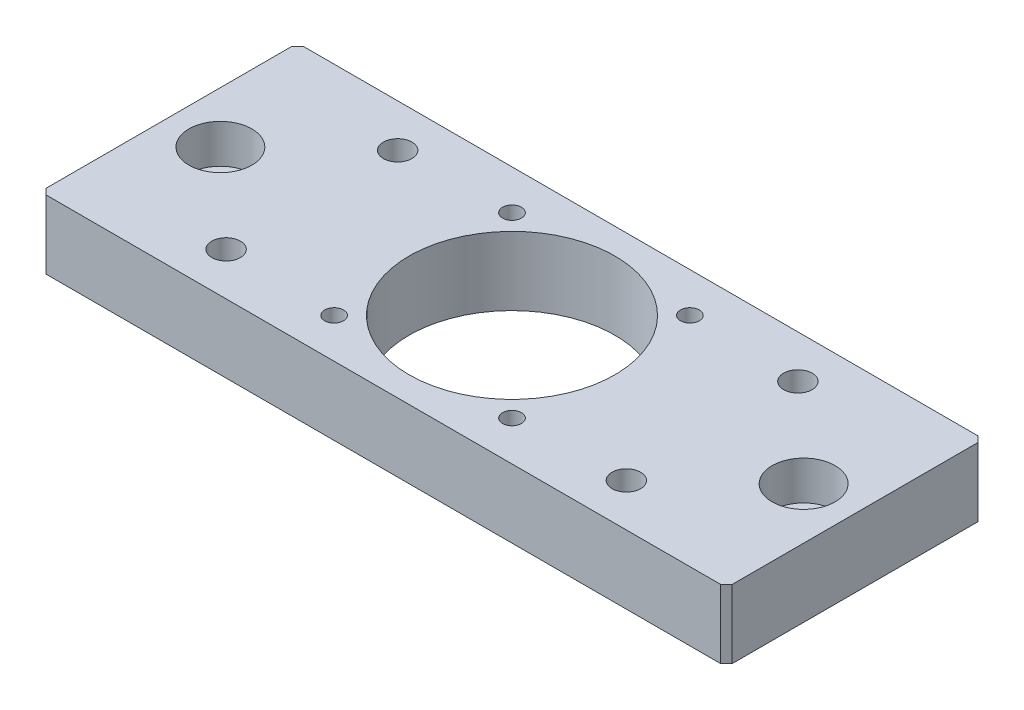
from build123d import *

# Parameters (mm, degrees)
SKETCH1_W                                            = 120
SKETCH1_H                                            = 45
BOSS_EXTRUDE1_DEPTH                                  = 12
CHAMFER1_SIZE                                        = 1
SKETCH2_R                                            = 18
CUT_EXTRUDE1_DEPTH                                   = 66.193941436
M4_TAPPED_HOLE1_D                                    = 3.3
HOLE_SIZE_PER_SOCKET_HEAD_CAP_SCREW_TYPE_D           = 6.6
HOLE_SIZE_PER_SOCKET_HEAD_CAP_SCREW_TYPE_CBORE_D     = 11
HOLE_SIZE_PER_SOCKET_HEAD_CAP_SCREW_TYPE_CBORE_DEPTH = 6.8
SKETCH7_R                                            = 6
CUT_EXTRUDE2_DEPTH                                   = 3.2
M4_TAPPED_HOLE2_D                                    = 3.3
M4_TAPPED_HOLE2_DEPTH                                = 11.5
M4_TAPPED_HOLE2_TIP                                  = 0.991420021
M6_TAPPED_HOLE1_D                                    = 5


with BuildPart() as part:
    # Sketch1 → Boss-Extrude1 (new body)
    with BuildSketch(Plane(origin=(0, 0, 0), x_dir=(1, 0, 0), z_dir=(0, 1, 0))):
        Rectangle(SKETCH1_W, SKETCH1_H)
    extrude(amount=BOSS_EXTRUDE1_DEPTH)

    # Chamfer1
    chamfer1_edges = [part.edges().sort_by_distance(p)[0] for p in [
        (-60, 6, -22.5),
        (60, 6, -22.5),
        (60, 6, 22.5),
        (-60, 6, 22.5),
    ]]
    chamfer(chamfer1_edges, length=CHAMFER1_SIZE)

    # Sketch2 → Cut-Extrude1 (cut, through all)
    with BuildSketch(Plane(origin=(0, 12, 0), x_dir=(1, 0, 0), z_dir=(0, 1, 0))):
        with Locations(Location((0, 0, 0), (0, 0, 270))):
            Circle(SKETCH2_R)
    extrude(amount=-CUT_EXTRUDE1_DEPTH, mode=Mode.SUBTRACT)

    # M4 Tapped Hole1 (through all)
    with Locations(Plane(origin=(0, 12, 0), x_dir=(-1, 0, 0), z_dir=(0, 1, 0))):
        with Locations((15.5565, -15.5565), (15.5565, 15.5565), (-15.5565, 15.5565), (-15.5565, -15.5565)):
            Hole(M4_TAPPED_HOLE1_D / 2)

    # Hole size per socket head cap screw type1 (through all)
    with Locations(Plane(origin=(0, 12, 0), x_dir=(-1, 0, 0), z_dir=(0, 1, 0))):
        with Locations((51, 0), (-51, 0)):
            CounterBoreHole(HOLE_SIZE_PER_SOCKET_HEAD_CAP_SCREW_TYPE_D / 2, HOLE_SIZE_PER_SOCKET_HEAD_CAP_SCREW_TYPE_CBORE_D / 2, HOLE_SIZE_PER_SOCKET_HEAD_CAP_SCREW_TYPE_CBORE_DEPTH)

    # Sketch7 → Cut-Extrude2 (cut)
    with BuildSketch(Plane.XZ):
        with Locations(Location((51, 0, 0), (0, 0, 270))):
            Circle(SKETCH7_R)
        with Locations(Location((-51, 0, 0), (0, 0, 270))):
            Circle(SKETCH7_R)
    extrude(amount=-CUT_EXTRUDE2_DEPTH, mode=Mode.SUBTRACT)

    # M4 Tapped Hole2
    with Locations(Plane(origin=(0, 0, -22.5), x_dir=(-1, 0, 0), z_dir=(0, 0, -1))):
        with Locations((-27.5, 7)):
            Hole(M4_TAPPED_HOLE2_D / 2, depth=M4_TAPPED_HOLE2_DEPTH)
            with Locations((0, 0, -(M4_TAPPED_HOLE2_DEPTH + M4_TAPPED_HOLE2_TIP / 2))):  # 118° drill point
                Cone(0, M4_TAPPED_HOLE2_D / 2, M4_TAPPED_HOLE2_TIP, mode=Mode.SUBTRACT)

    # M6 Tapped Hole1 (through all)
    with Locations(Plane(origin=(0, 12, 0), x_dir=(1, 0, 0), z_dir=(0, 1, 0))):
        with Locations((35, -15), (35, 15), (-35, -15), (-35, 15)):
            Hole(M6_TAPPED_HOLE1_D / 2)


solid = part.part
